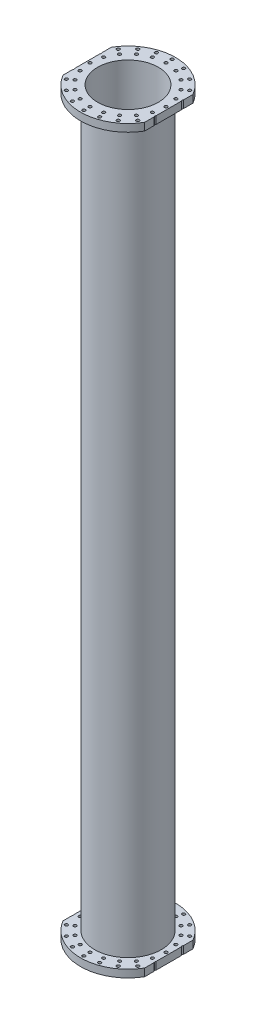
from build123d import *

# Parameters (mm, degrees)
SKETCH1_R                      = 160
BOSS_EXTRUDE1_DEPTH            = 40
SKETCH2_R                      = 175.5
SKETCH2_R_2                    = 160
BOSS_EXTRUDE2_DEPTH            = 3817
F_16_0_16_DIAMETER_HOLE1_D     = 16
F_16_0_16_DIAMETER_HOLE1_DEPTH = 40
LPATTERN1_COUNT                = 2
LPATTERN1_PITCH                = 3857


with BuildPart() as part:
    # Sketch1 → Boss-Extrude1 (new body)
    with BuildSketch(Plane(origin=(0, 0, 0), x_dir=(1, 0, 0), z_dir=(0, 1, 0))):
        with BuildLine():
            ThreePointArc((-215, -127.573508222), (0, -250), (215, -127.573508222))
            Line((215, -127.573508222), (215, 127.573508222))
            ThreePointArc((215, 127.573508222), (0, 250), (-215, 127.573508222))
            Line((-215, 127.573508222), (-215, -127.573508222))
        make_face()
        with Locations(Location((0, 0, 0), (0, 0, 270))):
            Circle(SKETCH1_R, mode=Mode.SUBTRACT)
    boss_extrude1 = extrude(amount=BOSS_EXTRUDE1_DEPTH)

    # Sketch2 → Boss-Extrude2 (add)
    with BuildSketch(Plane(origin=(0, 40, 0), x_dir=(1, 0, 0), z_dir=(0, 1, 0))):
        with Locations(Location((0, 0, 0), (0, 0, 270))):
            Circle(SKETCH2_R)
        with Locations(Location((0, 0, 0), (0, 0, 270))):
            Circle(SKETCH2_R_2, mode=Mode.SUBTRACT)
    extrude(amount=BOSS_EXTRUDE2_DEPTH)

    # Ø16.0 (16) Diameter Hole1
    with Locations(Plane(origin=(0, 40, 0), x_dir=(1, 0, 0), z_dir=(0, 1, 0))):
        with Locations((200, 0), (190.211303259, -61.803398875), (161.803398875, -117.557050458), (117.557050458, -161.803398875), (61.803398875, -190.211303259), (0, -200), (-61.803398875, -190.211303259), (-117.557050458, -161.803398875), (-161.803398875, -117.557050458), (-190.211303259, -61.803398875), (-200, 0), (-190.211303259, 61.803398875), (-161.803398875, 117.557050458), (-117.557050458, 161.803398875), (-61.803398875, 190.211303259), (0, 200), (61.803398875, 190.211303259), (117.557050458, 161.803398875), (161.803398875, 117.557050458), (190.211303259, 61.803398875), (232.5, 0), (221.120640039, -71.846451192), (188.096451192, -136.660071158), (136.660071158, -188.096451192), (71.846451192, -221.120640039), (0, -232.5), (-71.846451192, -221.120640039), (-136.660071158, -188.096451192), (-188.096451192, -136.660071158), (-221.120640039, -71.846451192), (-232.5, 0), (-221.120640039, 71.846451192), (-188.096451192, 136.660071158), (-136.660071158, 188.096451192), (-71.846451192, 221.120640039), (0, 232.5), (71.846451192, 221.120640039), (136.660071158, 188.096451192), (188.096451192, 136.660071158), (221.120640039, 71.846451192)):
            f_16_0_16_diameter_hole1 = Hole(F_16_0_16_DIAMETER_HOLE1_D / 2, depth=F_16_0_16_DIAMETER_HOLE1_DEPTH)

    # LPattern1: Boss-Extrude1, Ø16.0 (16) Diameter Hole1 ×2
    with Locations(*[(0, i * LPATTERN1_PITCH, 0) for i in range(1, LPATTERN1_COUNT)]):
        add(boss_extrude1)
        add(f_16_0_16_diameter_hole1, mode=Mode.SUBTRACT)


solid = part.part
